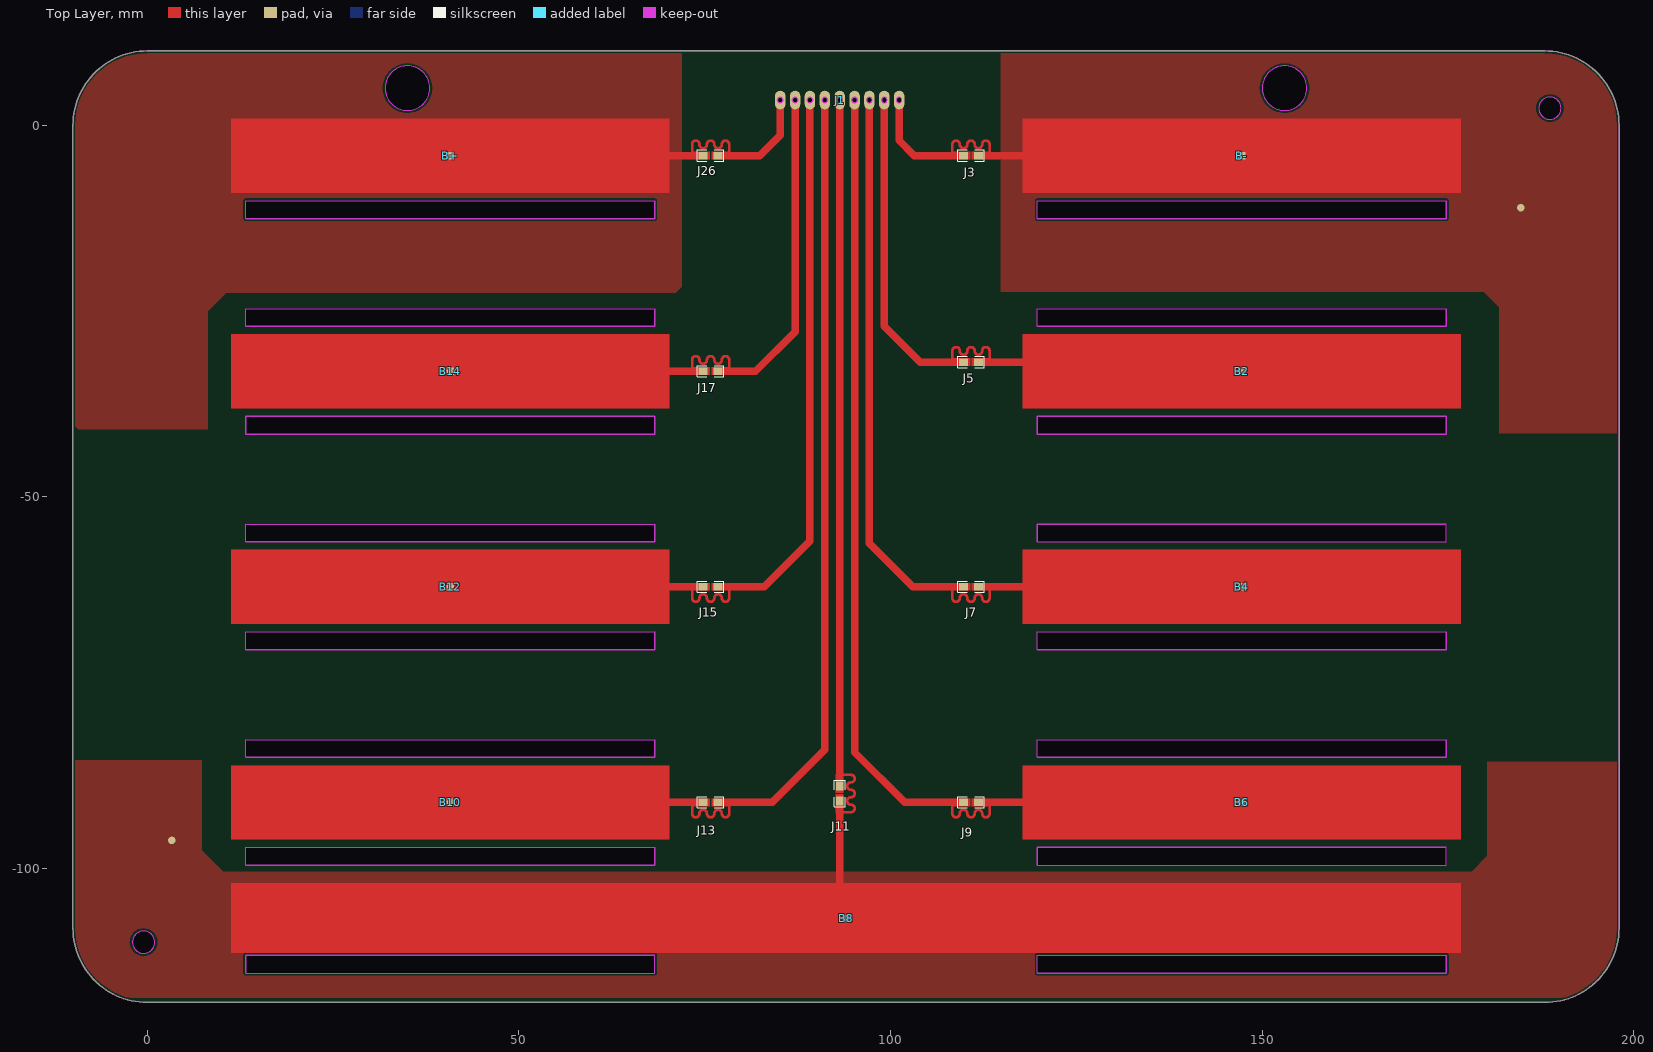
[diagram p0: Top Layer view]
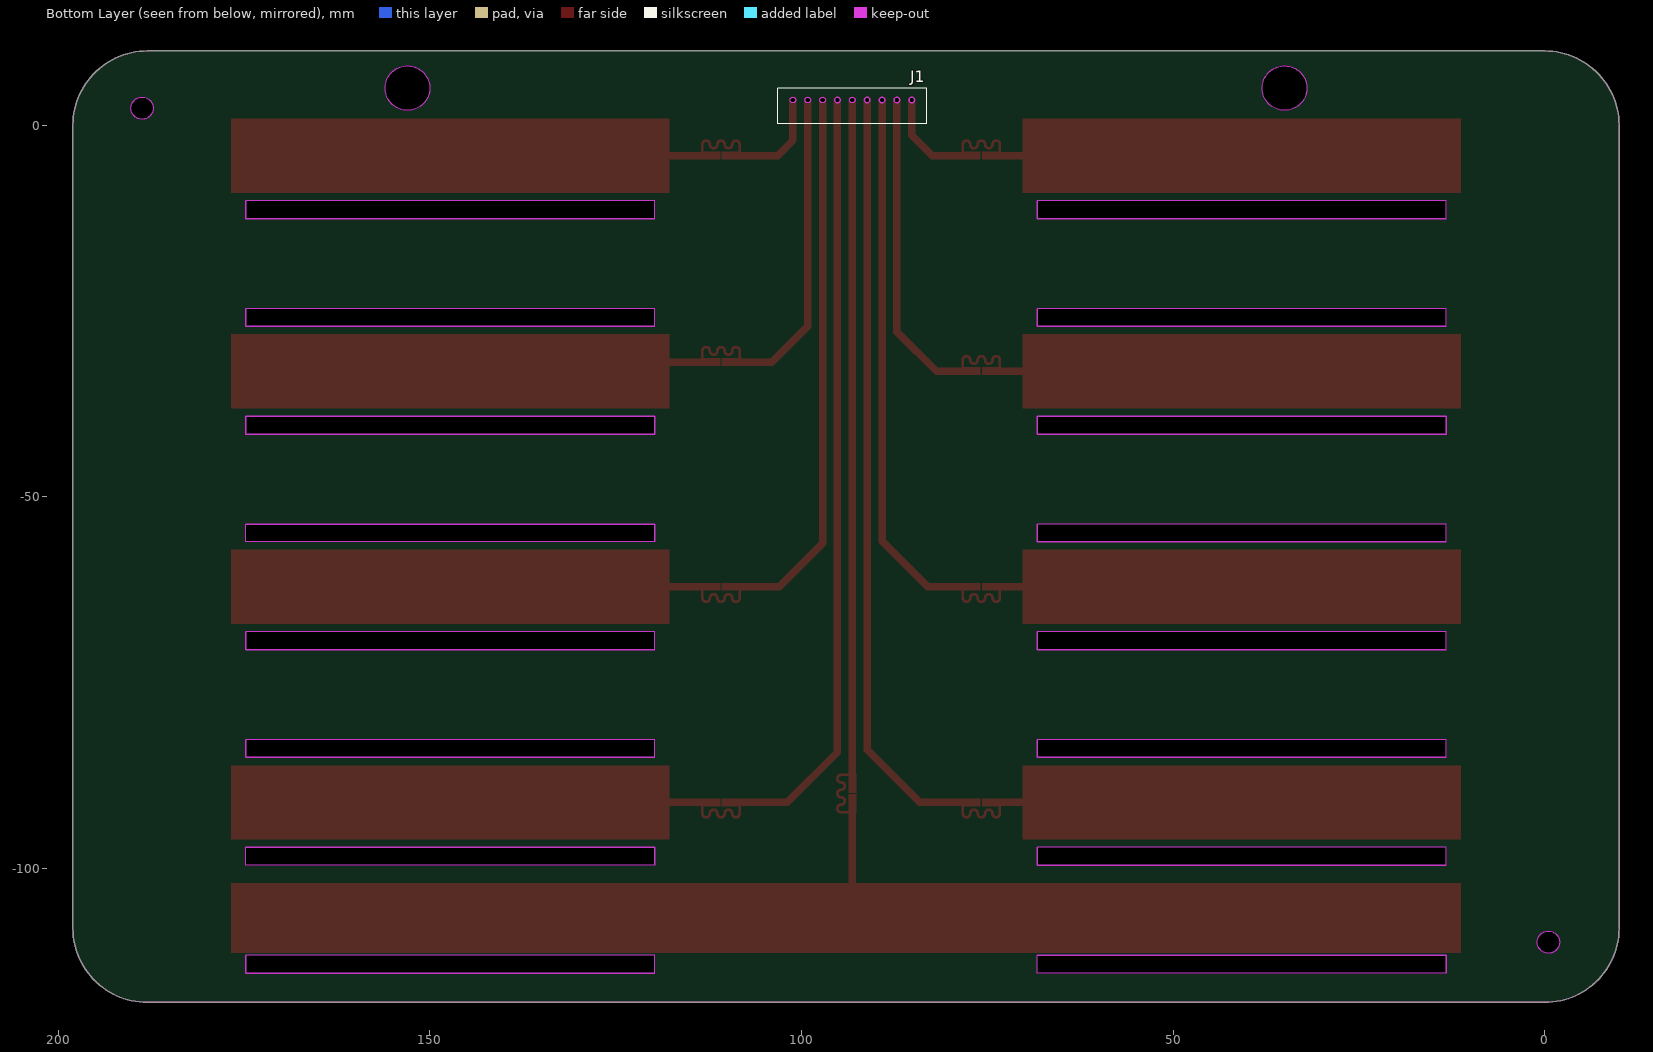
[diagram p1: Bottom Layer view, seen from below]
# Altium PCB MISC89348.PcbDoc
Units mm, origin at the board's own origin, x right, y up, seen from the top; angles counter-clockwise.
Board outline 208 x 128 mm, 2 copper layers (Top Layer, Bottom Layer); 19 components, 9 nets, 47 pads, 0 vias.

## Layer stack, top to bottom (the 12.6 mil dielectric is the usual default, probably not edited)
Top Solder: solder mask 0.0102, Solder Resist, Dk 3.5
Top Layer: signal copper 0.0356
Dielectric 1: dielectric 0.32, FR-4, Dk 4.8
Bottom Layer: signal copper 0.0356
Bottom Solder: solder mask 0.0102, Solder Resist, Dk 3.5

## Board outline
-10,-108 -10,0 cw(c0,0) 0,10 188,10 cw(c188,0) 198,0 198,-108 cw(c188,-108) 188,-118 0,-118 cw(c0,-108)
cut-out: 187.2,2.3 ccw(c188.7,2.3) 188.7,0.8 ccw(c188.7,2.3) 190.2,2.3 ccw(c188.7,2.3) 188.7,3.8 ccw(c188.7,2.3)
cut-out: 150,5 ccw(c153,5) 153,2 ccw(c153,5) 156,5 ccw(c153,5) 153,8 ccw(c153,5)
cut-out: 32,5 ccw(c35,5) 35,2 ccw(c35,5) 38,5 ccw(c35,5) 35,8 ccw(c35,5)
cut-out: -0.5,-111.4 ccw(c-0.5,-109.9) 1,-109.9 ccw(c-0.5,-109.9) -0.5,-108.4 ccw(c-0.5,-109.9) -2,-109.9 ccw(c-0.5,-109.9)
cut-out: 13.25,-12.55 13.25,-10.15 68.25,-10.15 68.25,-12.55
cut-out: 119.75,-12.55 119.75,-10.15 174.75,-10.15 174.75,-12.55
cut-out: 119.75,-27.05 119.75,-24.65 174.75,-24.65 174.75,-27.05
cut-out: 13.25,-27.05 13.25,-24.65 68.25,-24.65 68.25,-27.05
cut-out: 13.25,-41.55 13.25,-39.15 68.25,-39.15 68.25,-41.55
cut-out: 119.75,-41.55 119.75,-39.15 174.75,-39.15 174.75,-41.55
cut-out: 119.75,-56.05 174.75,-56.05 174.75,-53.65 119.75,-53.65
cut-out: 13.25,-56.05 13.25,-53.65 68.25,-53.65 68.25,-56.05
cut-out: 13.25,-70.55 13.25,-68.15 68.25,-68.15 68.25,-70.55
cut-out: 119.75,-70.55 119.75,-68.15 174.75,-68.15 174.75,-70.55
cut-out: 119.75,-85.05 119.75,-82.65 174.75,-82.65 174.75,-85.05
cut-out: 13.25,-85.05 13.25,-82.65 68.25,-82.65 68.25,-85.05
cut-out: 13.25,-99.55 13.25,-97.15 68.25,-97.15 68.25,-99.55
cut-out: 119.75,-99.55 174.75,-99.55 174.75,-97.15 119.75,-97.15
cut-out: 119.75,-114.05 119.75,-111.65 174.75,-111.65 174.75,-114.05
cut-out: 68.25,-114.05 68.25,-111.65 13.25,-111.65 13.25,-114.05
cut-out: 119.75,-12.55 119.75,-10.15 174.75,-10.15 174.75,-12.55
cut-out: 119.75,-41.55 174.75,-41.55 174.75,-39.15 119.75,-39.15
cut-out: 119.75,-70.55 119.75,-68.15 174.75,-68.15 174.75,-70.55
cut-out: 13.25,-12.55 13.25,-10.15 68.25,-10.15 68.25,-12.55
cut-out: 13.25,-41.55 68.25,-41.55 68.25,-39.15 13.25,-39.15
cut-out: 13.25,-85.05 13.25,-82.65 68.25,-82.65 68.25,-85.05

## Design rules (kind name [scope] priority, off if disabled: settings)
Clearance [All] p1: gap=0.3 ignorepadtopadclearanceinfootprint=FALSE
ComponentClearance [All] p1: gap=0 collisioncheckmode=3 verticalgap=0 showdistances=FALSE
HoleToHoleClearance [All] p1: gap=0 allowstackedmicrovias=TRUE
MinimumSolderMaskSliver [All] p1: minsoldermaskwidth=0
PolygonConnect [All] p1: connectstyle=Direct reliefconductorwidth=0.254 reliefentries=4 polygonreliefangle="90 Angle" airgapwidth=0.254
RoutingVias [All] p1: holewidth=0.711 width=1.27 viastyle="Through Hole" minholewidth=0.711 minwidth=1.27 maxholewidth=0.711 maxwidth=1.27
SilkToSilkClearance [All] p1: silktosilkclearance=0
SilkToSolderMaskClearance [IsPad] p1: minsilkscreentomaskgap=0 clearancetoexposedcopper=TRUE
SolderMaskExpansion [All] p1: expansion=0.102 istentingtop=FALSE
Width [All] p1: maxlimit=2 minlimit=0.254 preferedwidth=0.254 minimp=50.000000 maximp=50.000000 favimp=50.000000
25 further rules are at their usual default settings.

## Components (designator, comment, footprint, x,y, rotation, side; value= is the part's Value field where it differs from the comment)
B2 "Pth" 55*10*1MM 147.25,-33.1 r180 top locked
B4 "Pth" 55*10*1MM 147.25,-62.1 r180 top locked
B6 "Pth" 55*10*1MM 147.25,-91.1 r180 top locked
B8 "Pth" 161.5*10*1MM 94,-106.65 r180 top locked
B10 "Pth" 55*10*1MM 40.75,-91.1 r180 top locked
B12 "Pth" 55*10*1MM 40.75,-62.1 r180 top locked
B14 "Pth" 55*10*1MM 40.75,-33.1 r180 top locked
B+ "Pth" 55*10*1MM 40.75,-4.1 r180 top locked
B- "Pth" 55*10*1MM 147.25,-4.1 r180 top locked
J1 "HX-2.54mm-9P through-hole connector with latch" HX2.0-9P 93.15,3.4 r180 bottom locked
J3 "FPC" 异形电阻#1 110.814,-4.08 r90 top
J5 "FPC" 异形电阻#1 110.814,-31.859 r90 top
J7 "FPC" 异形电阻#1 110.814,-62.08 r270 top
J9 "FPC" 异形电阻#1 110.814,-91.08 r270 top
J11 "FPC" 异形电阻#2 93.15,-89.899 r0 top
J13 "FPC" 异形电阻#1 75.789,-91.08 r270 top
J15 "FPC" 异形电阻#1 75.789,-62.08 r270 top
J17 "FPC" 异形电阻#2 75.789,-33.08 r90 top
J26 "FPC" 异形电阻#2 75.789,-4.08 r90 top

## Footprints (in the part's own frame and the unit in brackets; to place one, negate y for a bottom-side part, rotate by r counter-clockwise, add the part's x,y. Pads: shape width x height; smd on the part's side, far side on the other; paste and mask are expansions set on the pad)
55*10*1MM [mm]
  rect 1x1 smd: 1(0,0)
  Top Layer region: -29.499,-5 29.501,-5 29.501,5 -29.499,5
161.5*10*1MM [mm]
  rect 1x1 smd: 1(0,0)
  Top Layer region: -82.749,-4.7 82.751,-4.7 82.751,4.7 -82.749,4.7
HX2.0-9P [mm]
  oval 1.4x2.5 smd far side: 1(-8,0) 2(-6,0) 3(-4,0) 4(-2,0) 5(0,0) 6(2,0) 7(4,0) 8(6,0) 9(8,0)
  round 0.75 hole 0.75: 1(-8,0) 2(-6,0) 3(-4,0) 4(-2,0) 5(0,0) 6(2,0) 7(4,0) 8(6,0) 9(8,0)
  Keep-Out Layer board cut-out: 6,-0.375 6.144,-0.346 6.265,-0.265 6.346,-0.144 6.375,0 6.375,0 6.346,0.144 6.265,0.265 6.144,0.346 6,0.375 6,0.375 5.856,0.346 5.735,0.265 5.654,0.144 5.625,0 5.625,0 5.654,-0.144 5.735,-0.265 5.856,-0.346 6,-0.375
  Keep-Out Layer board cut-out: 7.625,0 7.654,-0.144 7.735,-0.265 7.856,-0.346 8,-0.375 8,-0.375 8.144,-0.346 8.265,-0.265 8.346,-0.144 8.375,0 8.375,0 8.346,0.144 8.265,0.265 8.144,0.346 8,0.375 8,0.375 7.856,0.346 7.735,0.265 7.654,0.144 7.625,0
  Keep-Out Layer board cut-out: 3.625,0 3.654,-0.144 3.735,-0.265 3.856,-0.346 4,-0.375 4,-0.375 4.144,-0.346 4.265,-0.265 4.346,-0.144 4.375,0 4.375,0 4.346,0.144 4.265,0.265 4.144,0.346 4,0.375 4,0.375 3.856,0.346 3.735,0.265 3.654,0.144 3.625,0
  Keep-Out Layer board cut-out: 2,-0.375 2.144,-0.346 2.265,-0.265 2.346,-0.144 2.375,0 2.375,0 2.346,0.144 2.265,0.265 2.144,0.346 2,0.375 2,0.375 1.856,0.346 1.735,0.265 1.654,0.144 1.625,0 1.625,0 1.654,-0.144 1.735,-0.265 1.856,-0.346 2,-0.375
  Keep-Out Layer board cut-out: 0,-0.375 -0.144,-0.346 -0.265,-0.265 -0.346,-0.144 -0.375,0 -0.375,0 -0.346,0.144 -0.265,0.265 -0.144,0.346 0,0.375 0,0.375 0.144,0.346 0.265,0.265 0.346,0.144 0.375,0 0.375,0 0.346,-0.144 0.265,-0.265 0.144,-0.346 0,-0.375
  Keep-Out Layer board cut-out: -2,-0.375 -1.856,-0.346 -1.735,-0.265 -1.654,-0.144 -1.625,0 -1.625,0 -1.654,0.144 -1.735,0.265 -1.856,0.346 -2,0.375 -2,0.375 -2.144,0.346 -2.265,0.265 -2.346,0.144 -2.375,0 -2.375,0 -2.346,-0.144 -2.265,-0.265 -2.144,-0.346 -2,-0.375
  Keep-Out Layer board cut-out: -4,-0.375 -4.144,-0.346 -4.265,-0.265 -4.346,-0.144 -4.375,0 -4.375,0 -4.346,0.144 -4.265,0.265 -4.144,0.346 -4,0.375 -4,0.375 -3.856,0.346 -3.735,0.265 -3.654,0.144 -3.625,0 -3.625,0 -3.654,-0.144 -3.735,-0.265 -3.856,-0.346 -4,-0.375
  Keep-Out Layer board cut-out: -6,-0.375 -6.144,-0.346 -6.265,-0.265 -6.346,-0.144 -6.375,0 -6.375,0 -6.346,0.144 -6.265,0.265 -6.144,0.346 -6,0.375 -6,0.375 -5.856,0.346 -5.735,0.265 -5.654,0.144 -5.625,0 -5.625,0 -5.654,-0.144 -5.735,-0.265 -5.856,-0.346 -6,-0.375
  Keep-Out Layer board cut-out: -8,-0.375 -8.144,-0.346 -8.265,-0.265 -8.346,-0.144 -8.375,0 -8.375,0 -8.346,0.144 -8.265,0.265 -8.144,0.346 -8,0.375 -8,0.375 -7.856,0.346 -7.735,0.265 -7.654,0.144 -7.625,0 -7.625,0 -7.654,-0.144 -7.735,-0.265 -7.856,-0.346 -8,-0.375
  Keep-Out Layer circle w0.01: c0,0 r0.375
  Keep-Out Layer circle w0.01: c2,0 r0.375
  Keep-Out Layer circle w0.01: c4,0 r0.375
  Keep-Out Layer circle w0.01: c6,0 r0.375
  Keep-Out Layer circle w0.01: c8,0 r0.375
  Keep-Out Layer circle w0.01: c-2,0 r0.375
  Keep-Out Layer circle w0.01: c-4,0 r0.375
  Keep-Out Layer circle w0.01: c-6,0 r0.375
  Keep-Out Layer circle w0.01: c-8,0 r0.375
  silkscreen extent -10,-3.2 10,1.6
异形电阻#1 [mm]
  rect 1x1.2 smd mask+0: 1(0,1) 2(0,-1)
  Top Layer region: -0.5,-2.625 -0.496,-2.644 -0.485,-2.66 -0.469,-2.671 -0.45,-2.675 -0.45,-2.675 0.4,-2.675 0.438,-2.667 0.471,-2.646 0.492,-2.613 0.5,-2.575 0.5,-2.575 0.5,-0.125 -0.5,-0.125 -0.5,-0.125
  Top Layer region: 0.5,0.125 0.5,2.55 0.49,2.598 0.463,2.638 0.423,2.665 0.375,2.675 0.375,2.675 -0.425,2.675 -0.454,2.669 -0.478,2.653 -0.494,2.629 -0.5,2.6 -0.5,2.6 -0.5,0.125
  Top Layer pour cut-out: -1,3 2.5,3 2.5,-3 -1,-3
  Top Layer lines w0.2: -0.325,2.5 0,2.5
  Top Layer lines w0.35: -0.325,2.5 0,2.5 1.525,2.5 cw(c1.525,2) 1.525,1.5 ; 1.5,1.5 ccw(c1.5,1) 1.5,0.5 ; 1.525,0.5 cw(c1.525,0) 1.525,-0.5 ; 1.5,-0.5 ccw(c1.5,-1) 1.5,-1.5 ; 1.525,-1.5 cw(c1.525,-2) 1.525,-2.5 0,-2.5 -0.325,-2.5
  silkscreen extent -0.98,-2.04 0.95,2.03
异形电阻#2 [mm]
  rect 1x1.2 smd mask+0: 1(0,1) 2(0,-1)
  Top Layer region: -0.5,-2.625 -0.496,-2.644 -0.485,-2.66 -0.469,-2.671 -0.45,-2.675 -0.45,-2.675 0.4,-2.675 0.438,-2.667 0.471,-2.646 0.492,-2.613 0.5,-2.575 0.5,-2.575 0.5,-0.125 -0.5,-0.125 -0.5,-0.125
  Top Layer region: 0.5,0.125 0.5,2.55 0.49,2.598 0.463,2.638 0.423,2.665 0.375,2.675 0.375,2.675 -0.425,2.675 -0.454,2.669 -0.478,2.653 -0.494,2.629 -0.5,2.6 -0.5,2.6 -0.5,0.125
  Top Layer pour cut-out: -1,3 2.5,3 2.5,-3 -1,-3
  Top Layer lines w0.2: -0.325,2.5 -0.039,2.5 0,2.5
  Top Layer lines w0.35: -0.325,-2.5 0,-2.5 1.525,-2.5 ccw(c1.525,-2) 1.525,-1.5 ; -0.325,2.5 -0.039,2.5 0,2.5 1.525,2.5 cw(c1.525,2) 1.525,1.5 ; 1.5,-1.5 cw(c1.5,-1) 1.5,-0.5 ; 1.5,0.5 cw(c1.5,1) 1.5,1.5 ; 1.525,-0.5 ccw(c1.525,0) 1.525,0.5
  silkscreen extent -0.98,-2.04 0.95,2.03

## Part data
B2 B4 B6 B8 B10 B12 B14 B+ B-: "Through-hole pad"
J1: library part HX-2.54mm-9P直插带扣

## Free pads (board coordinates)
  round 1 smd: 3(3.3,-96.2) 3(184.789,-11.08)

## Nets (pads, with @x,y where several pads share a name; then routed paths per layer and width w, separated by ;. In a path a pad name is that pad's centre, name@x,y a point inside that pad or via, vN(x,y) a via of type N, cw(c..) or ccw(c..) an arc to the next point about the centre after c; other vN are vias at no path point)
B2: B2.1 J1.2 J5.1 J5.2 | length 79.1
  Top Layer w1: J1.2@99.15,3.4 99.15,-27.042 103.967,-31.859 108.314,-31.859 J5.1 ; J5.2 113.314,-31.859 146.009,-31.859 B2.1
B4: B4.1 J1.3 J7.1 J7.2 | length 110.2
  Top Layer w1: J1.3@97.15,3.4 97.15,-56.242 102.989,-62.08 108.314,-62.08 J7.2 ; J7.1 113.314,-62.08 147.23,-62.08 B4.1
B6: B6.1 J1.4 J9.1 J9.2 | length 140.5
  Top Layer w1: J1.4@95.15,3.4 95.15,-84.35 101.88,-91.08 108.314,-91.08 J9.2 ; J9.1@111.903,-91.1 B6.1
B8: B8.1 J1.5 J11.1 J11.2 pad.3@3.3,-96.2 | length 108.4
  Top Layer w1: J11.2 93.15,-92.399 93.15,-105.8 B8.1 ; J11.1 J1.5@93.15,3.4
B10: B10.1 J1.6 J13.1 J13.2 | length 138.8
  Top Layer w1: B10.1 73.289,-91.1 74.669,-91.1 74.689,-91.08 J13.2 ; J13.1 78.289,-91.08 84.089,-91.08 91.15,-84.019 J1.6@91.15,3.4
B12: B12.1 J1.7 J15.1 J15.2 | length 108.3
  Top Layer w1: B12.1 73.289,-62.1 74.669,-62.1 74.689,-62.08 J15.2 ; J15.1 78.289,-62.08 83.02,-62.08 89.15,-55.95 J1.7@89.15,3.4
B14: B14.1 J1.8 J17.1 J17.2 | length 77.8
  Top Layer w1: B14.1 73.289,-33.1 74.669,-33.1 74.689,-33.08 J17.1 ; J17.2 78.289,-33.08 81.82,-33.08 87.15,-27.75 J1.8@87.15,3.4
B+: B+.1 J1.9 J26.1 J26.2 | length 48.5
  Top Layer w1: B+.1 61.908,-4.1 ; 62.089,-4.28 61.908,-4.1 ; J26.1 74.689,-4.08 74.669,-4.1 73.289,-4.1 61.908,-4.1 ; J26.2 78.289,-4.08 82.42,-4.08 85.15,-1.35 J1.9@85.15,3.4
B-: B-.1 J1.1 J3.1 J3.2 pad.3@184.789,-11.08 | length 50.4
  Top Layer w1: J1.1@101.15,3.4 101.15,-2.042 103.189,-4.08 108.314,-4.08 J3.1 ; J3.2 113.314,-4.08 116.072,-4.08 116.092,-4.1 B-.1

## Polygon pours and split planes (outlines as drawn)
B- on Top Layer "NONET_L02_P-001" (solid, remove dead copper, pour order 1): 179.8,-22.4 181.9,-24.5 181.9,-41.4 197.9,-41.4 198.6,-40.7 198.6,8.6 197.1,10.1 114.8,9.998 114.8,-22.4
B+ on Top Layer "NONET_L02_P-001" (solid, remove dead copper, pour order 0): -9.9,-40.3 -9.3,-40.9 8.1,-40.9 8.1,-25 10.6,-22.5 31.4,-22.5 71.1,-22.5 71.9,-21.7 71.9,9.6 71.4,10.1 -9.9,10.1 -10,10 -9.9,9.9
B8 on Top Layer "NONET_L02_P-001" (solid, remove dead copper, pour order 2): 178.2,-100.4 180.3,-98.3 180.3,-85.6 197.9,-85.6 198.1,-85.8 198.1,-111.791 192.491,-117.4 -7.9,-117.4 -10,-115.3 -10,-85.9 -10.1,-85.8 -9.7,-85.4 7.3,-85.4 7.3,-97.5 10.2,-100.4

## Keep-outs
Keep-Out Layer:
  circle w0.1: c188.7,2.3 r1.5
  circle w0.1: c-0.5,-109.9 r1.5
  circle w0.013: c35,5 r3
  circle w0.013: c153,5 r3
  lines w0.013: -10,-108 ccw(c0,-108) 0,-118 188,-118 ccw(c188,-108) 198,-108 198,0 ccw(c188,0) 188,10 0,10 ccw(c0,0) -10,0 -10,-108 ; 13.25,-114.05 13.25,-111.65 68.25,-111.65 68.25,-114.05 13.25,-114.05 ; 13.25,-99.55 13.25,-97.15 68.25,-97.15 68.25,-99.55 13.25,-99.55 ; 13.25,-85.05 13.25,-82.65 68.25,-82.65 68.25,-85.05 13.25,-85.05 ; 13.25,-70.55 13.25,-68.15 68.25,-68.15 68.25,-70.55 13.25,-70.55 ; 13.25,-56.05 13.25,-53.65 68.25,-53.65 68.25,-56.05 13.25,-56.05 ; 13.25,-41.55 13.25,-39.15 68.25,-39.15 68.25,-41.55 13.25,-41.55 ; 13.25,-27.05 13.25,-24.65 68.25,-24.65 68.25,-27.05 13.25,-27.05 ; 13.25,-12.55 13.25,-10.15 68.25,-10.15 68.25,-12.55 13.25,-12.55 ; 119.75,-114.05 174.75,-114.05 174.75,-111.65 119.75,-111.65 119.75,-114.05 ; 119.75,-99.55 174.75,-99.55 174.75,-97.15 119.75,-97.15 119.75,-99.55 ; 119.75,-85.05 174.75,-85.05 174.75,-82.65 119.75,-82.65 119.75,-85.05 ; 119.75,-70.55 174.75,-70.55 174.75,-68.15 119.75,-68.15 119.75,-70.55 ; 119.75,-56.05 174.75,-56.05 174.75,-53.65 119.75,-53.65 119.75,-56.05 ; 119.75,-41.55 174.75,-41.55 174.75,-39.15 119.75,-39.15 119.75,-41.55 ; 119.75,-27.05 119.75,-24.65 174.75,-24.65 174.75,-27.05 119.75,-27.05 ; 119.75,-12.55 119.75,-10.15 174.75,-10.15 174.75,-12.55 119.75,-12.55

## Other copper
Top Layer:
  pour cut-out: 187.2,2.3 ccw(c188.7,2.3) 188.7,0.8 ccw(c188.7,2.3) 190.2,2.3 ccw(c188.7,2.3) 188.7,3.8 ccw(c188.7,2.3)
  pour cut-out: -2,-109.9 ccw(c-0.5,-109.9) -0.5,-111.4 ccw(c-0.5,-109.9) 1,-109.9 ccw(c-0.5,-109.9) -0.5,-108.4 ccw(c-0.5,-109.9)